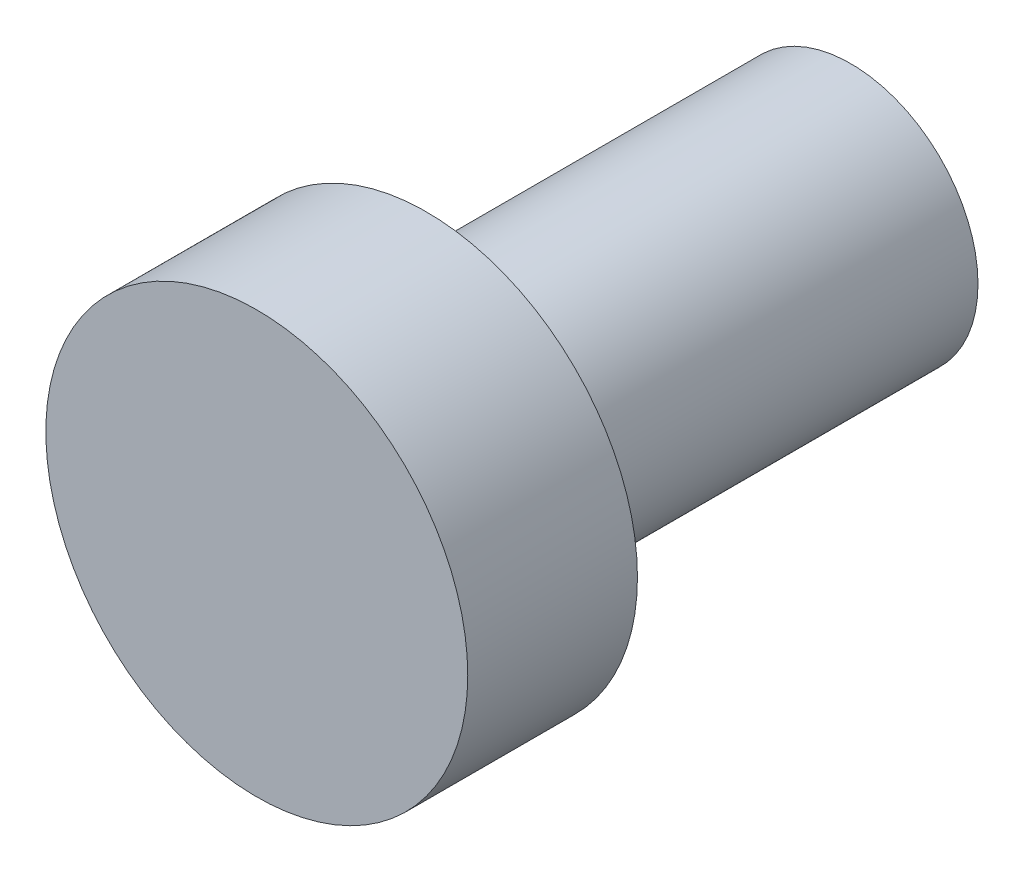
SolidWorks part; units mm, degrees
ref_plane "Front Plane" through (0, 0, 0) normal (0, 0, 1) x (1, 0, 0)
ref_plane "Top Plane" through (0, 0, 0) normal (0, 1, 0) x (1, 0, 0)
ref_plane "Right Plane" through (0, 0, 0) normal (1, 0, 0) x (0, 0, -1)
other "Configuration Table"
sketch "Sketch1" plane through (0, 0, 0) normal (0, 0, 1) x (1, 0, 0)
  circle A0 centre (-45.1978, 32.0258) radius 1.5
extrude "Boss-Extrude1" add sketch "Sketch1" against normal blind 5
sketch "Sketch2" plane through (0, 0, 0) normal (0, 0, 1) x (1, 0, 0)
  circle A0 centre (-45.1978, 32.0258) radius 2.4864
extrude "Boss-Extrude2" add sketch "Sketch2" along normal blind 2
